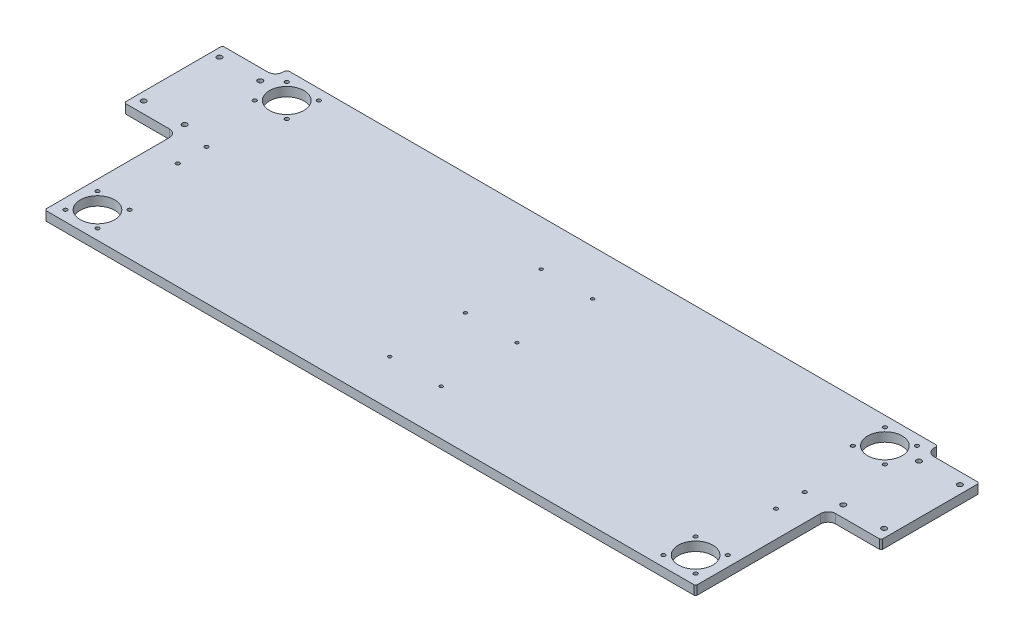
SolidWorks part; units mm, degrees
material "A6061"
ref_plane "前视基准面" through (0, 0, 0) normal (0, 0, 1) x (1, 0, 0)
ref_plane "上视基准面" through (0, 0, 0) normal (0, 1, 0) x (1, 0, 0)
ref_plane "右视基准面" through (0, 0, 0) normal (1, 0, 0) x (0, 0, -1)
sketch "草图1" plane through (0, 0, 0) normal (0, 0, 1) x (1, 0, 0)
  line L1 (500, 6) -> (-500, 6)
  line L2 (500, 6) -> (500, -6)
  line L3 (500, -6) -> (-500, -6)
  line L4 (-500, 6) -> (-500, -6)
  line L5 (500, 6) -> (-500, -6) construction
  line L6 (500, -6) -> (-500, 6) construction
  point P0 (0, 0)
  dimension "D1" = 1000
  dimension "D2" = 12
extrude "凸台-拉伸1" add sketch "草图1" along normal blind 320
hole_wizard "M5 螺纹孔1" positions "草图17" profile "草图18" tap size "M5" standard "GB" end condition through all
sketch "草图17" plane through (0, -6, 0) normal (0, -1, 0) x (-1, 0, 0)
  line L1 (0, 0) -> (0, -387.765) construction
  line L2 (500, 0) -> (-500, 0) construction
  point P36 (34, -260)
  point P37 (-34, -260)
  point P38 (34, -160)
  point P39 (-34, -160)
  point P40 (-34, -60)
  point P42 (34, -60)
  dimension "D1" = 100
  dimension "D2" = 68
  dimension "D4" = 100
  dimension "D6" = 60
sketch "草图18" plane through (-34, -6, 60) normal (1, 0, 0) x (0, 0, -1)
  line L0 (0, 0) -> (0, 12)
  line L1 (0, 12) -> (2.1, 12)
  line L2 (2.1, 12) -> (2.1, 0)
  line L5 (2.1, 0) -> (0, 0)
  line L11 (0, -6.35) -> (0, 107.95) construction
  dimension "通孔螺纹孔钻头直径" = 4.2
  dimension "通孔螺纹孔钻头深度" = 12
cosmetic thread "孔螺蚊线3" parameters "D2"=5
cosmetic thread "孔螺蚊线4" parameters "D2"=5
cosmetic thread "孔螺蚊线5" parameters "D2"=5
cosmetic thread "孔螺蚊线6" parameters "D2"=5
cosmetic thread "孔螺蚊线29" parameters "D2"=5
cosmetic thread "孔螺蚊线30" parameters "D2"=5
hole_wizard "Ø25.0 (45.5) 直径孔1" positions "草图19" profile "草图20" hole size "Ø25.0" standard "GB" end condition through all
sketch "草图19" plane through (0, 6, 0) normal (0, 1, 0) x (1, 0, 0)
  line L0 (0, -320) -> (0, 0) construction
  line L1 (500, -320) -> (-500, -320) construction
  line L5 (500, 0) -> (-500, 0) construction
  point P0 (395, -285)
  point P14 (395, -35)
  point P15 (-395, -35)
  point P16 (-395, -285)
  dimension "D1" = 790
  dimension "D2" = 250
  dimension "D3" = 35
sketch "草图20" plane through (395, 6, 285) normal (1, 0, 0) x (0, 0, 1)
  line L0 (0, 0) -> (0, 12)
  line L1 (0, 12) -> (22.75, 12)
  line L2 (22.75, 12) -> (22.75, 0)
  line L5 (22.75, 0) -> (0, 0)
  line L11 (0, -6.35) -> (0, 107.95) construction
  dimension "通孔孔直径" = 45.5
  dimension "通孔孔深度" = 12
sketch "草图22" plane through (0, -6, 0) normal (0, -1, 0) x (1, 0, 0)
  line L0 (0, 0) -> (0, 400.4552) construction
  line L1 (500, 320) -> (430, 320)
  line L2 (500, 320) -> (500, 145)
  line L3 (500, 145) -> (440, 145)
  line L4 (430, 320) -> (430, 155)
  line L5 (-430, 320) -> (-430, 155)
  line L6 (-500, 145) -> (-440, 145)
  line L7 (-500, 320) -> (-500, 145)
  line L8 (-500, 320) -> (-430, 320)
  line L10 (-430, 0) -> (-430, 5)
  line L11 (500, 0) -> (430, 0)
  line L12 (500, 0) -> (500, 15)
  line L13 (500, 15) -> (440, 15)
  line L14 (430, 0) -> (430, 5)
  line L15 (-500, 15) -> (-440, 15)
  line L16 (-500, 0) -> (-500, 15)
  line L17 (-500, 0) -> (-430, 0)
  arc A0 (440, 145) -> (430, 155) centre (440, 155) cw
  arc A1 (-440, 145) -> (-430, 155) centre (-440, 155) ccw
  arc A2 (440, 15) -> (430, 5) centre (440, 5) ccw
  arc A3 (-440, 15) -> (-430, 5) centre (-440, 5) cw
  dimension "D1" = 10
  dimension "D2" = 10
  dimension "D3" = 70
  dimension "D4" = 130
  dimension "D5" = 15
extrude "切除-拉伸2" cut sketch "草图22" against normal up to surface (12 mm away) up to face at (395, 6, 307.75)
hole_wizard "打孔尺寸(%根据)内六角圆柱头螺钉的类型2" positions "草图12" profile "草图13" counterbore size "M6" standard "GB" end condition through all
sketch "草图12" plane through (0, -6, 0) normal (0, 1, 0) x (1, 0, 0)
  line L0 (0, 0) -> (0, -127.5724) construction
  line L5 (500, -80) -> (421.0849, -80) construction
  line L6 (500, -145) -> (500, -15) construction
  point P12 (489, -130)
  point P15 (489, -30)
  point P18 (435, -30)
  point P21 (435, -130)
  point P33 (-435, -130)
  point P34 (-435, -30)
  point P35 (-489, -30)
  point P36 (-489, -130)
  dimension "D1" = 924
  dimension "D2" = 54
  dimension "D3" = 100
sketch "草图13" plane through (489, -6, 130) normal (1, 0, 0) x (0, 0, -1)
  line L0 (0, 0) -> (0, 12)
  line L1 (0, 12) -> (3.3, 12)
  line L3 (3.3, 12) -> (3.3, 6.8)
  line L4 (3.3, 6.8) -> (5.5, 6.8)
  line L5 (5.5, 6.8) -> (5.5, 0)
  line L7 (5.5, 0) -> (0, 0)
  line L11 (0, -6.35) -> (0, 107.95) construction
  dimension "通孔孔直径" = 6.6
  dimension "通孔孔深度" = 12
  dimension "柱形沉头孔直径" = 11
  dimension "柱形沉头孔深度" = 6.8
chamfer "倒角1" distance 2 angle 45 8 edges at (-430, 0, 320) (-500, 0, 145) (430, 0, 320) (500, 0, 145) (-500, 0, 15) (-430, 0, 0) (500, 0, 15) (430, 0, 0)
hole_wizard "M6 螺纹孔1" positions "草图23" profile "草图24" tap size "M6" standard "GB" end condition through all
sketch "草图23" plane through (0, 6, 0) normal (0, 1, 0) x (1, 0, 0)
  line L0 (0, 0) -> (0, -341.9972) construction
  line L3 (-395, -35) -> (-395, -285) construction
  line L5 (-395, -160) -> (-317.081, -160) construction
  point P0 (-395, -141)
  point P2 (-395, -179)
  point P10 (395, -179)
  point P11 (395, -141)
  dimension "D1" = 38
  dimension "D3" = 790
sketch "草图24" plane through (-395, 6, 141) normal (1, 0, 0) x (0, 0, 1)
  line L0 (0, 0) -> (0, 12)
  line L1 (0, 12) -> (2.5, 12)
  line L2 (2.5, 12) -> (2.5, 0)
  line L5 (2.5, 0) -> (0, 0)
  line L11 (0, -6.35) -> (0, 107.95) construction
  dimension "通孔螺纹孔钻头直径" = 5
  dimension "通孔螺纹孔钻头深度" = 12
cosmetic thread "孔螺蚊线9" parameters "D2"=6
cosmetic thread "孔螺蚊线10" parameters "D2"=6
cosmetic thread "孔螺蚊线11" parameters "D2"=6
cosmetic thread "孔螺蚊线12" parameters "D2"=6
hole_wizard "M6 螺纹孔2" positions "草图25" profile "草图26" tap size "M6" standard "GB" end condition through all
sketch "草图25" plane through (0, -6, 0) normal (0, -1, 0) x (-1, 0, 0)
  line L0 (0, 0) -> (0, -320) construction
  line L1 (428, -320) -> (-428, -320) construction
  circle A0 centre (-395, -285) radius 30 construction
  circle A1 centre (395, -285) radius 30 construction
  circle A2 centre (395, -35) radius 30 construction
  circle A3 centre (-395, -35) radius 30 construction
  point P0 (-416.2132, -263.7868)
  point P6 (-373.7868, -263.7868)
  point P7 (-373.7868, -306.2132)
  point P8 (-416.2132, -306.2132)
  point P24 (373.7868, -263.7868)
  point P25 (416.2132, -263.7868)
  point P26 (416.2132, -306.2132)
  point P27 (373.7868, -306.2132)
  point P30 (373.7868, -13.7868)
  point P31 (416.2132, -13.7868)
  point P32 (416.2132, -56.2132)
  point P33 (373.7868, -56.2132)
  point P36 (-416.2132, -13.7868)
  point P37 (-373.7868, -13.7868)
  point P38 (-373.7868, -56.2132)
  point P39 (-416.2132, -56.2132)
  dimension "D2" = 60
  dimension "D1" = 4
sketch "草图26" plane through (416.2132, -6, 263.7868) normal (1, 0, 0) x (0, 0, -1)
  line L0 (0, 0) -> (0, 12)
  line L1 (0, 12) -> (2.5, 12)
  line L2 (2.5, 12) -> (2.5, 0)
  line L5 (2.5, 0) -> (0, 0)
  line L11 (0, -6.35) -> (0, 107.95) construction
  dimension "通孔螺纹孔钻头直径" = 5
  dimension "通孔螺纹孔钻头深度" = 12
cosmetic thread "孔螺蚊线13" parameters "D2"=6
cosmetic thread "孔螺蚊线14" parameters "D2"=6
cosmetic thread "孔螺蚊线15" parameters "D2"=6
cosmetic thread "孔螺蚊线16" parameters "D2"=6
cosmetic thread "孔螺蚊线17" parameters "D2"=6
cosmetic thread "孔螺蚊线18" parameters "D2"=6
cosmetic thread "孔螺蚊线19" parameters "D2"=6
cosmetic thread "孔螺蚊线20" parameters "D2"=6
cosmetic thread "孔螺蚊线21" parameters "D2"=6
cosmetic thread "孔螺蚊线22" parameters "D2"=6
cosmetic thread "孔螺蚊线23" parameters "D2"=6
cosmetic thread "孔螺蚊线24" parameters "D2"=6
cosmetic thread "孔螺蚊线25" parameters "D2"=6
cosmetic thread "孔螺蚊线26" parameters "D2"=6
cosmetic thread "孔螺蚊线27" parameters "D2"=6
cosmetic thread "孔螺蚊线28" parameters "D2"=6
